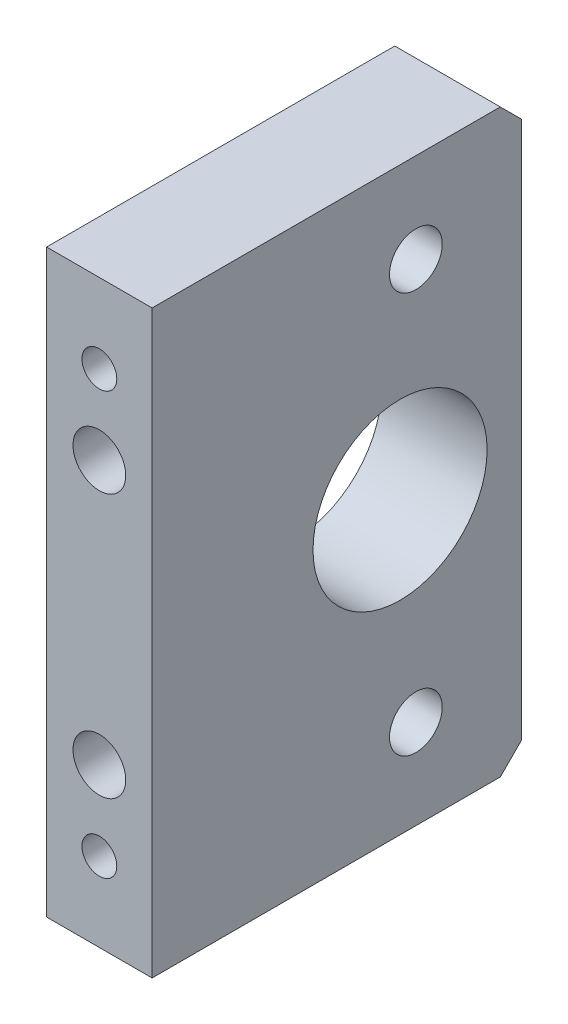
from build123d import *

# Parameters (mm, degrees)
SKETCH_1_W                = 35
SKETCH_1_H                = 55
EXTRUDE_1_DEPTH           = 10
SKETCH_2_R                = 8.25
CUT_EXTRUDE_1_DEPTH       = 110
HOLE_WIZARD_M6_1_D        = 5
HOLE_WIZARD_M4_1_D        = 3.3
HOLE_WIZARD_M4_1_DEPTH    = 10.1
HOLE_WIZARD_M4_1_TIP      = 0.991420021
HOLE_WIZARD_5_0_5_1_D     = 5
HOLE_WIZARD_5_0_5_1_DEPTH = 10.1
HOLE_WIZARD_5_0_5_1_TIP   = 1.502151548
CHAMFER_1_SIZE            = 2


with BuildPart() as part:
    # 草图1 → 凸台-拉伸1 (new body)
    with BuildSketch(Plane(origin=(0, 0, 0), x_dir=(0, 0, -1), z_dir=(1, 0, 0))):
        Rectangle(SKETCH_1_W, SKETCH_1_H)
    extrude(amount=EXTRUDE_1_DEPTH)

    # 草图2 → 切除-拉伸1 (cut)
    with BuildSketch(Plane.ZY):
        with Locations((-6, 0)):
            Circle(SKETCH_2_R)
    extrude(amount=-CUT_EXTRUDE_1_DEPTH, mode=Mode.SUBTRACT)

    # M6 螺纹孔1 (through all)
    with Locations(Plane.ZY):
        with Locations((-7.5, -19)):
            hole_wizard_m6_1 = Hole(HOLE_WIZARD_M6_1_D / 2)

    # 镜向1: M6 螺纹孔1 across plane
    add(hole_wizard_m6_1.mirror(Plane.ZX), mode=Mode.SUBTRACT)

    # M4 螺纹孔1
    with Locations(Plane.XY.offset(17.5)):
        with Locations((5, 20), (5, -20)):
            Hole(HOLE_WIZARD_M4_1_D / 2, depth=HOLE_WIZARD_M4_1_DEPTH)
            with Locations((0, 0, -(HOLE_WIZARD_M4_1_DEPTH + HOLE_WIZARD_M4_1_TIP / 2))):  # 118° drill point
                Cone(0, HOLE_WIZARD_M4_1_D / 2, HOLE_WIZARD_M4_1_TIP, mode=Mode.SUBTRACT)

    # Ø5.0 (5) 直径孔1
    with Locations(Plane.XY.offset(17.5)):
        with Locations((5, 12.5), (5, -12.5)):
            Hole(HOLE_WIZARD_5_0_5_1_D / 2, depth=HOLE_WIZARD_5_0_5_1_DEPTH)
            with Locations((0, 0, -(HOLE_WIZARD_5_0_5_1_DEPTH + HOLE_WIZARD_5_0_5_1_TIP / 2))):  # 118° drill point
                Cone(0, HOLE_WIZARD_5_0_5_1_D / 2, HOLE_WIZARD_5_0_5_1_TIP, mode=Mode.SUBTRACT)

    # 倒角1
    chamfer_1_edges = [part.edges().sort_by_distance(p)[0] for p in [
        (5, -27.5, -17.5),
        (5, 27.5, -17.5),
    ]]
    chamfer(chamfer_1_edges, length=CHAMFER_1_SIZE)


solid = part.part
